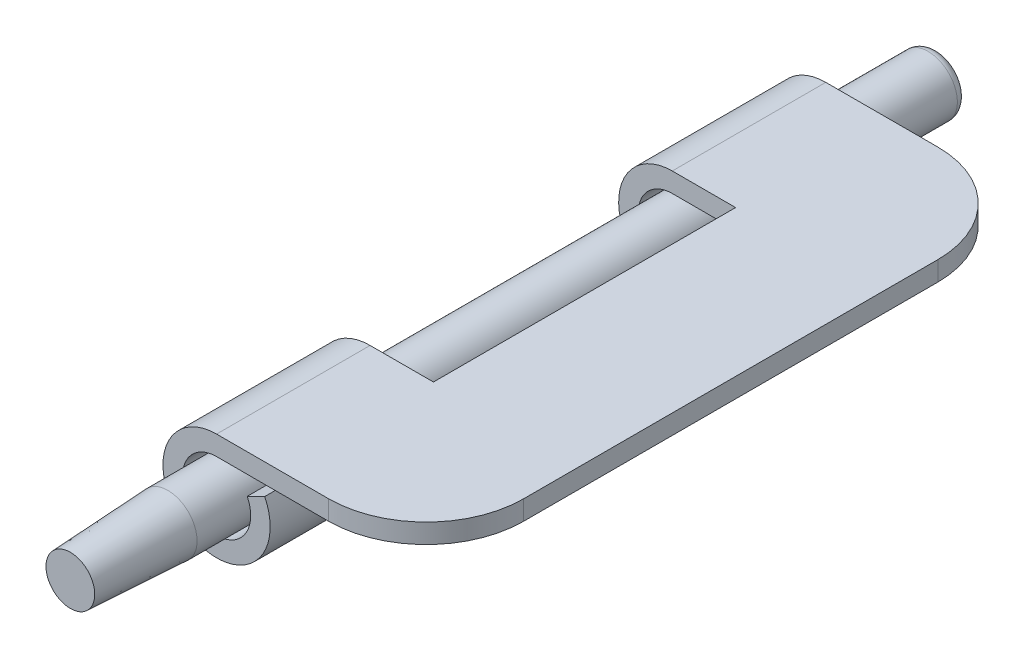
from build123d import *

# Parameters (mm, degrees)
EXTRUDE_5_DEPTH     = 31.25
SKETCH_4_W          = 12
SKETCH_4_H          = 31
CUT_EXTRUDE_1_DEPTH = 40.494461637
SKETCH_8_R          = 3
EXTRUDE_4_DEPTH     = 89
CHAMFER_2_SIZE      = 0.5
CHAMFER_2_SIZE2     = 10
FILLET_1_R          = 10
FILLET_2_R          = 1


with BuildPart() as part:
    # 草图3 → 拉伸-薄壁5 (new, symmetric)
    with BuildSketch(Plane.XY):
        with BuildLine():
            Line((21.5, 0), (0, 0))
            ThreePointArc((0, 0), (-1.852031969, -6.469844707), (3.142998481, -1.960012809))
            Line((3.142998481, -1.960012809), (4.938997613, -1.080020128))
            ThreePointArc((4.938997613, -1.080020128), (-2.910335952, -8.166898826), (0, 2))
            Line((0, 2), (21.5, 2))
            Line((21.5, 2), (21.5, 0))
        make_face()
    extrude(amount=EXTRUDE_5_DEPTH, both=True)

    # 草图4 → 切除-拉伸1 (cut, through all)
    with BuildSketch(Plane(origin=(0, 2, 0), x_dir=(1, 0, 0), z_dir=(0, 1, 0))):
        with Locations((0.5, 0)):
            Rectangle(SKETCH_4_W, SKETCH_4_H)
    extrude(amount=-CUT_EXTRUDE_1_DEPTH, mode=Mode.SUBTRACT)

    # 圆角1
    fillet_1_edges = [part.edges().sort_by_distance(p)[0] for p in [
        (21.5, 1, 31.25),
        (21.5, 1, -31.25),
    ]]
    fillet(fillet_1_edges, radius=FILLET_1_R)


with BuildPart() as body_2:
    # 草图8 → 凸台-拉伸4 (new body)
    with BuildSketch(Plane(origin=(0, 0, -42.75), x_dir=(-1, 0, 0), z_dir=(0, 0, -1))):
        with Locations((0, -3.5)):
            Circle(SKETCH_8_R)
    extrude(amount=-EXTRUDE_4_DEPTH)

    # 倒角2
    chamfer_2_edges = [body_2.edges().sort_by_distance(p)[0] for p in [
        (3, -3.5, 46.25),
    ]]
    chamfer_2_side = [body_2.faces().sort_by_distance(p)[0] for p in [
        (0, -3.5, 46.25),
    ]]
    chamfer(chamfer_2_edges, length=CHAMFER_2_SIZE, length2=CHAMFER_2_SIZE2, reference=chamfer_2_side[0])

    # 圆角2
    fillet_2_edges = [body_2.edges().sort_by_distance(p)[0] for p in [
        (3, -3.5, -42.75),
    ]]
    fillet(fillet_2_edges, radius=FILLET_2_R)


solid = Compound([part.part, body_2.part])
